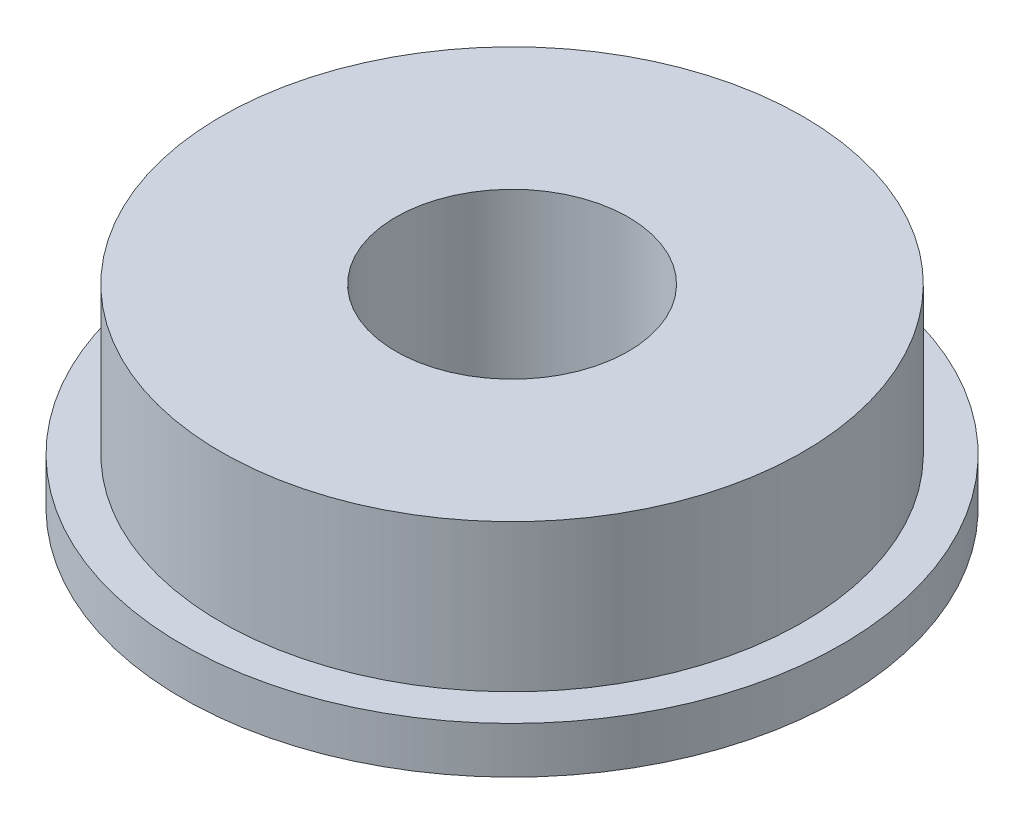
from build123d import *


with BuildPart() as part:
    # 草图1 → 旋转1 (revolve)
    with BuildSketch(Plane.XY, mode=Mode.PRIVATE) as revolve_1_sk:
        Polygon((3, 4.599056604), (3, -0.400943396), (8.5, -0.400943396), (8.5, 0.799056604), (7.5, 0.799056604), (7.5, 4.599056604), align=None)
    revolve(revolve_1_sk.sketch.rotate(Axis((0, 0, 0), (0, 1, 0)), 90), axis=Axis((0, 0, 0), (0, 1, 0)))


solid = part.part
